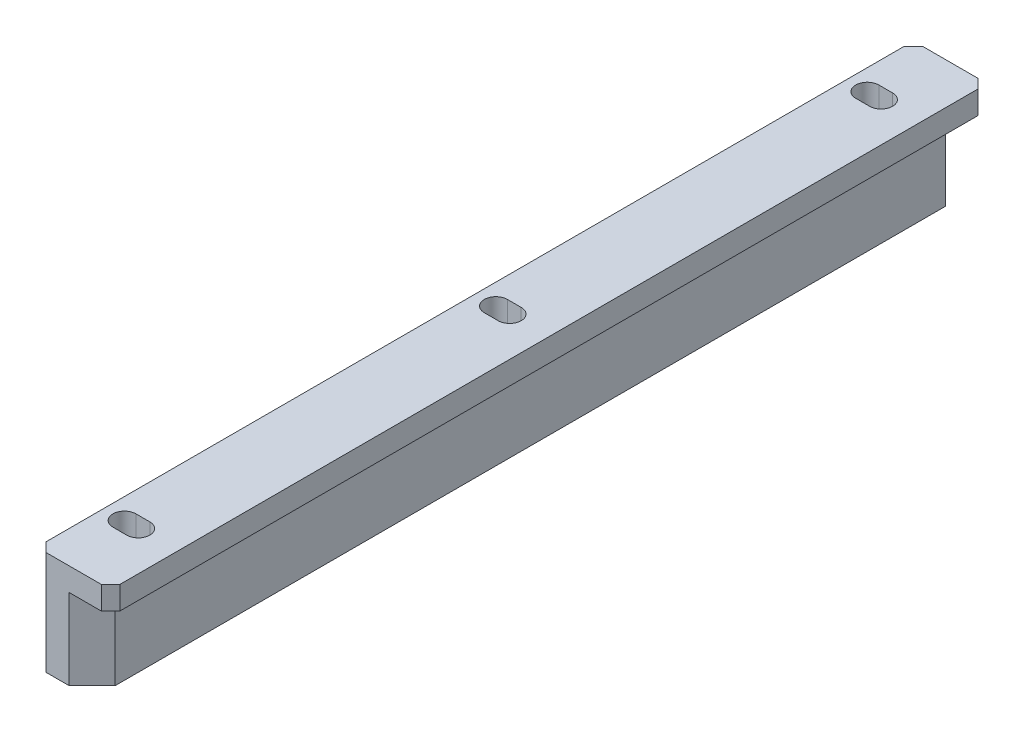
SolidWorks part; units mm, degrees
ref_plane "前视基准面" through (0, 0, 0) normal (0, 0, 1) x (1, 0, 0)
ref_plane "上视基准面" through (0, 0, 0) normal (0, 1, 0) x (1, 0, 0)
ref_plane "右视基准面" through (0, 0, 0) normal (1, 0, 0) x (0, 0, -1)
sketch "草图1" plane through (0, 0, 0) normal (0, 0, 1) x (1, 0, 0)
  line L0 (0, 0) -> (0, 22.5)
  line L1 (0, 22.5) -> (16, 22.5)
  line L2 (16, 22.5) -> (16, 17.5)
  line L3 (16, 17.5) -> (12, 17.5)
  line L4 (12, 17.5) -> (12, 0)
  line L5 (12, 0) -> (0, 0)
  dimension "D1" = 17.5
  dimension "D2" = 5
  dimension "D3" = 4
  dimension "D4" = 12
extrude "凸台-拉伸1" add sketch "草图1" along normal mid plane 190
chamfer "倒角1" distance 5 angle 45 2 edges at (12, 8.75, -95) (12, 8.75, 95)
chamfer "倒角2" distance 2 angle 45 4 edges at (0, 11.25, 95) (0, 11.25, -95) (16, 20, -95) (16, 20, 95)
sketch "草图2" plane through (0, 0, 0) normal (0, -1, 0) x (1, 0, 0)
  line L0 (4.5, 80.5) -> (7.5, 80.5) construction
  line L1 (4.5, 83) -> (7.5, 83)
  line L2 (4.5, 78) -> (7.5, 78)
  line L3 (0, 93) -> (0, -93) construction
  line L4 (2, 95) -> (7, 95) construction
  line L5 (4.5, 0) -> (7.5, 0) construction
  line L6 (4.5, 2.5) -> (7.5, 2.5)
  line L7 (4.5, -2.5) -> (7.5, -2.5)
  line L8 (0, 0) -> (12, 0) construction
  line L9 (12, 90) -> (12, -90) construction
  line L10 (4.5, -80.5) -> (7.5, -80.5) construction
  line L11 (4.5, -83) -> (7.5, -83)
  line L12 (4.5, -78) -> (7.5, -78)
  arc A0 (4.5, 83) -> (4.5, 78) centre (4.5, 80.5) ccw
  arc A1 (7.5, 78) -> (7.5, 83) centre (7.5, 80.5) ccw
  arc A2 (4.5, 2.5) -> (4.5, -2.5) centre (4.5, 0) ccw
  arc A3 (7.5, -2.5) -> (7.5, 2.5) centre (7.5, 0) ccw
  arc A4 (4.5, -83) -> (4.5, -78) centre (4.5, -80.5) cw
  arc A5 (7.5, -78) -> (7.5, -83) centre (7.5, -80.5) cw
  point P2 (6, 80.5)
  point P13 (6, 0)
  point P25 (6, -80.5)
  dimension "D1" = 2.5
  dimension "D2" = 3
  dimension "D3" = 6
  dimension "D4" = 12
  dimension "D5" = 3
extrude "切除-拉伸1" cut sketch "草图2" against normal up to next
